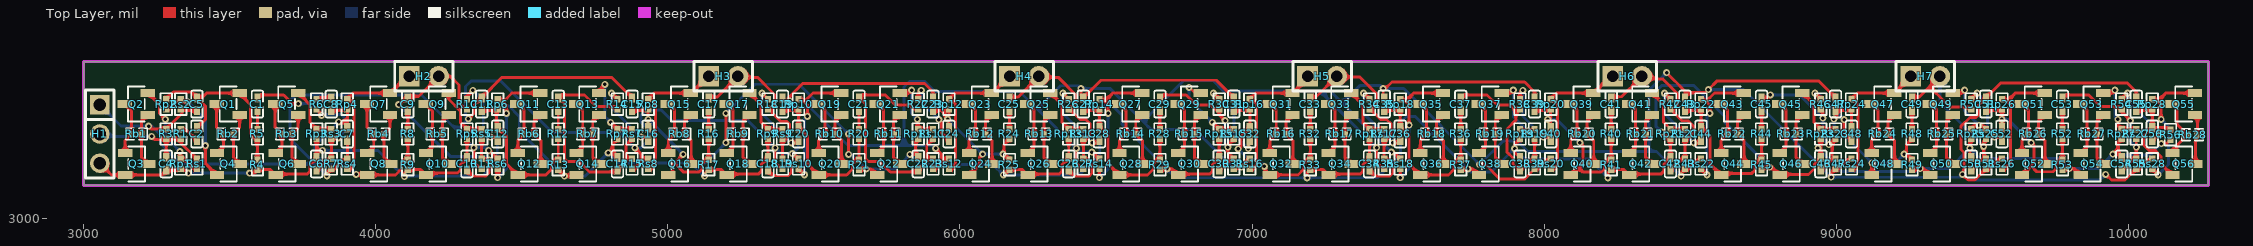
[diagram p0: Top Layer view]
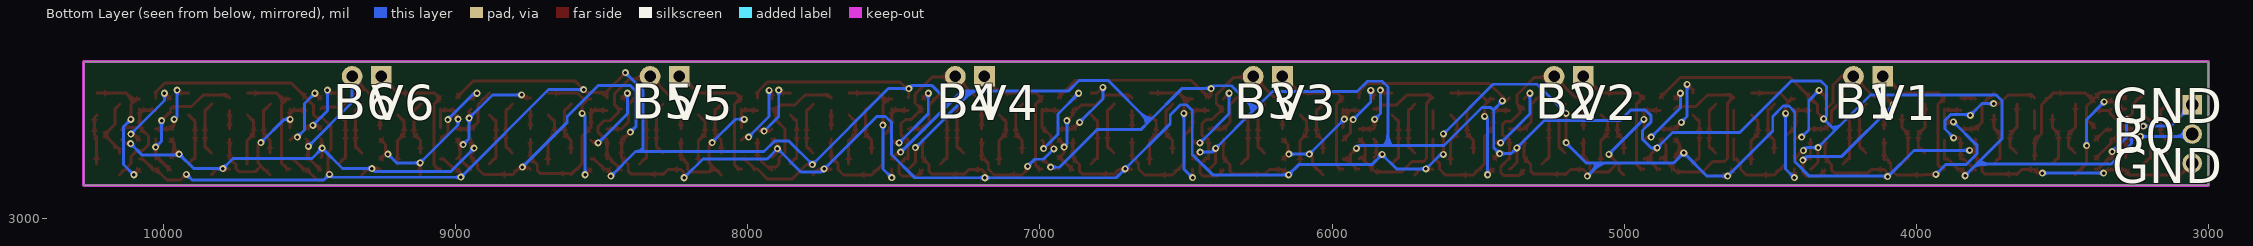
[diagram p1: Bottom Layer view, seen from below]
# Altium PCB MISC51432.pcbdoc (part 1 of 2)
Units mil, origin at the board's own origin, x right, y up, seen from the top; angles counter-clockwise.
Board outline 7274.02 x 423.7 mil, 2 copper layers (Top Layer, Bottom Layer), stack 62.206 mil thick; 257 components, 141 nets, 571 pads, 133 vias.

## Layer stack, top to bottom
Top Solder Mask Layer: solder mask 0.394, Dk 3.3
Top Layer: signal copper 1.379
Dielectric1: surface 59.449, FR4, Dk 4.5
Bottom Layer: signal copper 1.378
Bottom Solder Mask Layer: solder mask 0.394, Dk 3.3

## Board outline
3000,3536.14 3000,3112.44 10274.02,3112.44 10274.02,3536.14

## Design rules (kind name [scope] priority, off if disabled: settings)
BoardOutlineClearance copperThickness2oz_1 [All] p2 off: genericclearance=7.99 ignorepadtopadclearanceinfootprint=FALSE except(0: Arc-SplitContinuation Track-SplitContinuation SMDPad-SplitContinuation THPad-SplitContinuation Via-SplitContinuation Fill-SplitContinuation Region-SplitContinuation Poly-SplitContinuation Text-SplitContinuation Hole-SplitContinuation; 5.98: Arc-CutoutEdge Track-CutoutEdge SMDPad-CutoutEdge THPad-CutoutEdge Via-CutoutEdge Text-CutoutEdge; 6.9: Hole-OutlineEdge Hole-CutoutEdge; 10: Poly-OutlineEdge Poly-CutoutEdge; 11.81: Arc-OutlineEdge Track-OutlineEdge SMDPad-OutlineEdge THPad-OutlineEdge Via-OutlineEdge Fill-OutlineEdge Region-OutlineEdge Text-OutlineEdge Fill-CutoutEdge Region-CutoutEdge)
BoardOutlineClearance Plane_innerPlane_1 [All] p4 off: genericclearance=4.02 ignorepadtopadclearanceinfootprint=FALSE except(0: Arc-SplitContinuation Track-SplitContinuation SMDPad-SplitContinuation THPad-SplitContinuation Via-SplitContinuation Fill-SplitContinuation Region-SplitContinuation Poly-SplitContinuation Text-SplitContinuation Hole-SplitContinuation; 5.98: Arc-CutoutEdge Track-CutoutEdge SMDPad-CutoutEdge THPad-CutoutEdge Via-CutoutEdge Text-CutoutEdge; 6.9: Hole-OutlineEdge Hole-CutoutEdge; 10: Poly-OutlineEdge Poly-CutoutEdge; 11.81: Arc-OutlineEdge Track-OutlineEdge SMDPad-OutlineEdge THPad-OutlineEdge Via-OutlineEdge Fill-OutlineEdge Region-OutlineEdge Text-OutlineEdge Fill-CutoutEdge Region-CutoutEdge)
BoardOutlineClearance Copper_copperRegion_1 [All] p6 off: genericclearance=4.02 ignorepadtopadclearanceinfootprint=FALSE except(0: Arc-SplitContinuation Track-SplitContinuation SMDPad-SplitContinuation THPad-SplitContinuation Via-SplitContinuation Fill-SplitContinuation Region-SplitContinuation Poly-SplitContinuation Text-SplitContinuation Hole-SplitContinuation; 5.98: Arc-CutoutEdge Track-CutoutEdge SMDPad-CutoutEdge THPad-CutoutEdge Via-CutoutEdge Text-CutoutEdge; 6.9: Hole-OutlineEdge Hole-CutoutEdge; 10: Poly-OutlineEdge Poly-CutoutEdge; 11.81: Arc-OutlineEdge Track-OutlineEdge SMDPad-OutlineEdge THPad-OutlineEdge Via-OutlineEdge Fill-OutlineEdge Region-OutlineEdge Text-OutlineEdge Fill-CutoutEdge Region-CutoutEdge)
BoardOutlineClearance copperThickness1oz_1 [All] p8: genericclearance=4.02 ignorepadtopadclearanceinfootprint=FALSE except(0: Arc-SplitContinuation Track-SplitContinuation SMDPad-SplitContinuation THPad-SplitContinuation Via-SplitContinuation Fill-SplitContinuation Region-SplitContinuation Poly-SplitContinuation Text-SplitContinuation Hole-SplitContinuation; 5.98: Arc-CutoutEdge Track-CutoutEdge SMDPad-CutoutEdge THPad-CutoutEdge Via-CutoutEdge Text-CutoutEdge; 6.9: Hole-OutlineEdge Hole-CutoutEdge; 10: Poly-OutlineEdge Poly-CutoutEdge; 11.81: Arc-OutlineEdge Track-OutlineEdge SMDPad-OutlineEdge THPad-OutlineEdge Via-OutlineEdge Fill-OutlineEdge Region-OutlineEdge Text-OutlineEdge Fill-CutoutEdge Region-CutoutEdge)
Clearance copperThickness2oz [All] p1 off: gap=7.99 ignorepadtopadclearanceinfootprint=FALSE except(5.98: SMDPad-Track SMDPad-SMDPad THPad-Track SMDPad-THPad THPad-THPad Track-Via SMDPad-Via THPad-Via Via-Via Fill-SMDPad Region-SMDPad Fill-THPad Region-THPad Fill-Via Region-Via Fill-Fill Fill-Region Region-Region Arc-Track Arc-SMDPad Arc-THPad Arc-Via Fill-Arc Region-Arc Arc-Arc Text-Track SMDPad-Text Text-THPad Text-Via Fill-Text Region-Text Arc-Text Text-Text; 6.9: Hole-Track Hole-SMDPad Hole-THPad Hole-Via Fill-Hole Region-Hole Hole-Arc Hole-Text; 10: Poly-Track Poly-SMDPad Poly-THPad Poly-Via Poly-Fill Poly-Region Poly-Poly Poly-Arc Poly-Text Poly-Hole; 11.81: Fill-Track Region-Track)
Clearance Plane_innerPlane [All] p3 off: gap=4.02 ignorepadtopadclearanceinfootprint=FALSE except(5.98: SMDPad-Track SMDPad-SMDPad THPad-Track SMDPad-THPad THPad-THPad Track-Via SMDPad-Via THPad-Via Via-Via Fill-SMDPad Region-SMDPad Fill-THPad Region-THPad Fill-Via Region-Via Fill-Fill Fill-Region Region-Region Arc-Track Arc-SMDPad Arc-THPad Arc-Via Fill-Arc Region-Arc Arc-Arc Text-Track SMDPad-Text Text-THPad Text-Via Fill-Text Region-Text Arc-Text Text-Text; 6.9: Hole-Track Hole-SMDPad Hole-THPad Hole-Via Fill-Hole Region-Hole Hole-Arc Hole-Text; 10: Poly-Track Poly-SMDPad Poly-THPad Poly-Via Poly-Fill Poly-Region Poly-Poly Poly-Arc Poly-Text Poly-Hole; 11.81: Fill-Track Region-Track)
Clearance Copper_copperRegion [All] p5 off: gap=4.02 ignorepadtopadclearanceinfootprint=FALSE except(5.98: SMDPad-Track SMDPad-SMDPad THPad-Track SMDPad-THPad THPad-THPad Track-Via SMDPad-Via THPad-Via Via-Via Fill-SMDPad Region-SMDPad Fill-THPad Region-THPad Fill-Via Region-Via Fill-Fill Fill-Region Region-Region Arc-Track Arc-SMDPad Arc-THPad Arc-Via Fill-Arc Region-Arc Arc-Arc Text-Track SMDPad-Text Text-THPad Text-Via Fill-Text Region-Text Arc-Text Text-Text; 6.9: Hole-Track Hole-SMDPad Hole-THPad Hole-Via Fill-Hole Region-Hole Hole-Arc Hole-Text; 10: Poly-Track Poly-SMDPad Poly-THPad Poly-Via Poly-Fill Poly-Region Poly-Poly Poly-Arc Poly-Text Poly-Hole; 11.81: Fill-Track Region-Track)
Clearance copperThickness1oz [All] p7: gap=4.02 ignorepadtopadclearanceinfootprint=FALSE except(5.98: SMDPad-Track SMDPad-SMDPad THPad-Track SMDPad-THPad THPad-THPad Track-Via SMDPad-Via THPad-Via Via-Via Fill-SMDPad Region-SMDPad Fill-THPad Region-THPad Fill-Via Region-Via Fill-Fill Fill-Region Region-Region Arc-Track Arc-SMDPad Arc-THPad Arc-Via Fill-Arc Region-Arc Arc-Arc Text-Track SMDPad-Text Text-THPad Text-Via Fill-Text Region-Text Arc-Text Text-Text; 6.9: Hole-Track Hole-SMDPad Hole-THPad Hole-Via Fill-Hole Region-Hole Hole-Arc Hole-Text; 10: Poly-Track Poly-SMDPad Poly-THPad Poly-Via Poly-Fill Poly-Region Poly-Poly Poly-Arc Poly-Text Poly-Hole; 11.81: Fill-Track Region-Track)
DiffPairsRouting differentialPair [All] p1: maxlimit=6 minlimit=6 mostfreqgap=6 toplayer_minwidth=5 toplayer_prefwidth=10 toplayer_maxwidth=100 toplayer_mingap=6 toplayer_prefgap=6 toplayer_maxgap=6 bottomlayer_minwidth=5 bottomlayer_prefwidth=10 bottomlayer_maxwidth=100 bottomlayer_mingap=6 bottomlayer_prefgap=6 bottomlayer_maxgap=6 maxuncoupledlength=10
HoleToHoleClearance otherClearance [All] p1: gap=11.81 allowstackedmicrovias=TRUE
Length netLength [All] p1: minlimit=0 maxlimit=0
PasteMaskExpansion pasteMaskExpansion [All] p1: expansion=0
PlaneConnect innerPlane [All] p1: planeconnectstyle=Relief reliefexpansion=20 reliefentries=4 reliefconductorwidth=10 reliefairgap=10
PolygonConnect copperRegion [All] p1: connectstyle=Relief reliefconductorwidth=10 reliefentries=4 polygonreliefangle="90 Angle" airgapwidth=10 via.connectstyle=Relief via.reliefconductorwidth=10 via.reliefentries=4 via.polygonreliefangle="90 Angle" via.airgapwidth=10
RoutingVias viaSize [All] p1: holewidth=12.01 width=24.02 viastyle="Through Hole" minholewidth=11.81 minwidth=19.68 maxholewidth=248.03 maxwidth=393.7
SolderMaskExpansion solderMaskExpansion [IsVia] p1: expansion=-1000 istentingtop=TRUE
SolderMaskExpansion solderMaskExpansion [All] p2: expansion=2 istentingtop=FALSE
Width copperThickness2oz_2 [All] p1 off: maxlimit=100 minlimit=8 preferedwidth=10
Width copperThickness1oz_2 [All] p2: maxlimit=100 minlimit=5 preferedwidth=10

## Components (designator, comment, footprint, x,y, rotation, side; value= is the part's Value field where it differs from the comment)
C1 "0.1uF" C0402 3594.62,3391.14 r270 top
C2 "0.1uF" C0402 3387.5,3288.64 r270 top
C4 "0.1uF" C0402 3282.5,3186.14 r90 top
C5 "0.1uF" C0402 3387.5,3391.14 r270 top
C6 "0.1uF" C0402 3797.5,3186.14 r270 top
C7 "0.1uF" C0402 3902.5,3288.64 r270 top
C8 "0.1uF" C0402 3847.5,3391.14 r90 top
C9 "0.1uF" C0402 4109.62,3391.14 r270 top
C10 "0.1uF" C0402 4312.5,3186.14 r270 top
C11 "0.1uF" C0402 4362.5,3391.14 r90 top
C12 "0.1uF" C0402 4417.5,3288.64 r270 top
C13 "0.1uF" C0402 4624.62,3391.14 r270 top
C14 "0.1uF" C0402 4827.5,3186.14 r270 top
C15 "0.1uF" C0402 4877.5,3391.14 r90 top
C16 "0.1uF" C0402 4932.5,3288.64 r270 top
C17 "0.1uF" C0402 5139.62,3391.14 r270 top
C18 "0.1uF" C0402 5342.5,3186.14 r270 top
C19 "0.1uF" C0402 5392.5,3391.14 r90 top
C20 "0.1uF" C0402 5447.5,3288.64 r270 top
C21 "0.1uF" C0402 5654.62,3391.14 r270 top
C22 "0.1uF" C0402 5857.5,3186.14 r270 top
C23 "0.1uF" C0402 5907.5,3391.14 r90 top
C24 "0.1uF" C0402 5962.5,3288.64 r270 top
C25 "0.1uF" C0402 6169.62,3391.14 r270 top
C26 "0.1uF" C0402 6372.5,3186.14 r270 top
C27 "0.1uF" C0402 6422.5,3391.14 r90 top
C28 "0.1uF" C0402 6477.5,3288.64 r270 top
C29 "0.1uF" C0402 6684.62,3391.14 r270 top
C30 "0.1uF" C0402 6887.5,3186.14 r270 top
C31 "0.1uF" C0402 6937.5,3391.14 r90 top
C32 "0.1uF" C0402 6992.5,3288.64 r270 top
C33 "0.1uF" C0402 7199.62,3391.14 r270 top
C34 "0.1uF" C0402 7402.5,3186.14 r270 top
C35 "0.1uF" C0402 7452.5,3391.14 r90 top
C36 "0.1uF" C0402 7507.5,3288.64 r270 top
C37 "0.1uF" C0402 7714.62,3391.14 r270 top
C38 "0.1uF" C0402 7917.5,3186.14 r270 top
C39 "0.1uF" C0402 7967.5,3391.14 r90 top
C40 "0.1uF" C0402 8022.5,3288.64 r270 top
C41 "0.1uF" C0402 8229.62,3391.14 r270 top
C42 "0.1uF" C0402 8432.5,3186.14 r270 top
C43 "0.1uF" C0402 8482.5,3391.14 r90 top
C44 "0.1uF" C0402 8537.5,3288.64 r270 top
C45 "0.1uF" C0402 8744.62,3391.14 r270 top
C46 "0.1uF" C0402 8947.5,3186.14 r270 top
C47 "0.1uF" C0402 8997.5,3391.14 r90 top
C48 "0.1uF" C0402 9052.5,3288.64 r270 top
C49 "0.1uF" C0402 9259.62,3391.14 r270 top
C50 "0.1uF" C0402 9462.5,3186.14 r270 top
C51 "0.1uF" C0402 9512.5,3391.14 r90 top
C52 "0.1uF" C0402 9567.5,3288.64 r270 top
C53 "0.1uF" C0402 9774.62,3391.14 r270 top
C54 "0.1uF" C0402 9977.5,3186.14 r270 top
C55 "0.1uF" C0402 10027.5,3391.14 r90 top
C56 "0.1uF" C0402 10082.5,3288.64 r270 top
H1 "" HDR-TH_3P-P2.54-V-M 3055,3288.64 r270 top
H2 "" HDR-TH_2P-P2.54-V-M-1 4165,3486.14 r0 top
H3 "" HDR-TH_2P-P2.54-V-M-1 5190,3486.14 r0 top
H4 "" HDR-TH_2P-P2.54-V-M-1 6220,3486.14 r0 top
H5 "" HDR-TH_2P-P2.54-V-M-1 7240,3486.14 r0 top
H6 "" HDR-TH_2P-P2.54-V-M-1 8285,3486.14 r0 top
H7 "" HDR-TH_2P-P2.54-V-M-1 9305,3486.14 r0 top
Q1 "MMBT3906" SOT-23-3_L2.9-W1.3-P1.90-LS2.4-BR 3494.31,3391.14 r0 top
Q2 "MMBT3904" SOT-23-3_L2.9-W1.3-P1.90-LS2.4-BR 3180,3391.14 r0 top
Q3 "MMBT3906" SOT-23-3_L2.9-W1.3-P1.90-LS2.4-BR 3181.38,3186.14 r180 top
Q4 "MMBT3904" SOT-23-3_L2.9-W1.3-P1.90-LS2.4-BR 3495.69,3186.14 r180 top
Q5 "MMBT3904" SOT-23-3_L2.9-W1.3-P1.90-LS2.4-BR 3695,3391.14 r0 top
Q6 "MMBT3906" SOT-23-3_L2.9-W1.3-P1.90-LS2.4-BR 3696.38,3186.14 r180 top
Q7 "MMBT3904" SOT-23-3_L2.9-W1.3-P1.90-LS2.4-BR 4009.31,3391.14 r0 top
Q8 "MMBT3906" SOT-23-3_L2.9-W1.3-P1.90-LS2.4-BR 4010.69,3186.14 r180 top
Q9 "MMBT3904" SOT-23-3_L2.9-W1.3-P1.90-LS2.4-BR 4210,3391.14 r0 top
Q10 "MMBT3906" SOT-23-3_L2.9-W1.3-P1.90-LS2.4-BR 4211.38,3186.14 r180 top
Q11 "MMBT3904" SOT-23-3_L2.9-W1.3-P1.90-LS2.4-BR 4524.31,3391.14 r0 top
Q12 "MMBT3906" SOT-23-3_L2.9-W1.3-P1.90-LS2.4-BR 4525.69,3186.14 r180 top
Q13 "MMBT3904" SOT-23-3_L2.9-W1.3-P1.90-LS2.4-BR 4725,3391.14 r0 top
Q14 "MMBT3906" SOT-23-3_L2.9-W1.3-P1.90-LS2.4-BR 4726.38,3186.14 r180 top
Q15 "MMBT3904" SOT-23-3_L2.9-W1.3-P1.90-LS2.4-BR 5039.31,3391.14 r0 top
Q16 "MMBT3906" SOT-23-3_L2.9-W1.3-P1.90-LS2.4-BR 5040.69,3186.14 r180 top
Q17 "MMBT3904" SOT-23-3_L2.9-W1.3-P1.90-LS2.4-BR 5240,3391.14 r0 top
Q18 "MMBT3906" SOT-23-3_L2.9-W1.3-P1.90-LS2.4-BR 5241.38,3186.14 r180 top
Q19 "MMBT3904" SOT-23-3_L2.9-W1.3-P1.90-LS2.4-BR 5554.31,3391.14 r0 top
Q20 "MMBT3906" SOT-23-3_L2.9-W1.3-P1.90-LS2.4-BR 5555.69,3186.14 r180 top
Q21 "MMBT3904" SOT-23-3_L2.9-W1.3-P1.90-LS2.4-BR 5755,3391.14 r0 top
Q22 "MMBT3906" SOT-23-3_L2.9-W1.3-P1.90-LS2.4-BR 5756.38,3186.14 r180 top
Q23 "MMBT3904" SOT-23-3_L2.9-W1.3-P1.90-LS2.4-BR 6069.31,3391.14 r0 top
Q24 "MMBT3906" SOT-23-3_L2.9-W1.3-P1.90-LS2.4-BR 6070.69,3186.14 r180 top
Q25 "MMBT3904" SOT-23-3_L2.9-W1.3-P1.90-LS2.4-BR 6270,3391.14 r0 top
Q26 "MMBT3906" SOT-23-3_L2.9-W1.3-P1.90-LS2.4-BR 6271.38,3186.14 r180 top
Q27 "MMBT3904" SOT-23-3_L2.9-W1.3-P1.90-LS2.4-BR 6584.31,3391.14 r0 top
Q28 "MMBT3906" SOT-23-3_L2.9-W1.3-P1.90-LS2.4-BR 6585.69,3186.14 r180 top
Q29 "MMBT3904" SOT-23-3_L2.9-W1.3-P1.90-LS2.4-BR 6785,3391.14 r0 top
Q30 "MMBT3906" SOT-23-3_L2.9-W1.3-P1.90-LS2.4-BR 6786.38,3186.14 r180 top
Q31 "MMBT3904" SOT-23-3_L2.9-W1.3-P1.90-LS2.4-BR 7099.31,3391.14 r0 top
Q32 "MMBT3906" SOT-23-3_L2.9-W1.3-P1.90-LS2.4-BR 7100.69,3186.14 r180 top
Q33 "MMBT3904" SOT-23-3_L2.9-W1.3-P1.90-LS2.4-BR 7300,3391.14 r0 top
Q34 "MMBT3906" SOT-23-3_L2.9-W1.3-P1.90-LS2.4-BR 7301.38,3186.14 r180 top
Q35 "MMBT3904" SOT-23-3_L2.9-W1.3-P1.90-LS2.4-BR 7614.31,3391.14 r0 top
Q36 "MMBT3906" SOT-23-3_L2.9-W1.3-P1.90-LS2.4-BR 7615.69,3186.14 r180 top
Q37 "MMBT3904" SOT-23-3_L2.9-W1.3-P1.90-LS2.4-BR 7815,3391.14 r0 top
Q38 "MMBT3906" SOT-23-3_L2.9-W1.3-P1.90-LS2.4-BR 7816.38,3186.14 r180 top
Q39 "MMBT3904" SOT-23-3_L2.9-W1.3-P1.90-LS2.4-BR 8129.31,3391.14 r0 top
Q40 "MMBT3906" SOT-23-3_L2.9-W1.3-P1.90-LS2.4-BR 8130.69,3186.14 r180 top
Q41 "MMBT3904" SOT-23-3_L2.9-W1.3-P1.90-LS2.4-BR 8330,3391.14 r0 top
Q42 "MMBT3906" SOT-23-3_L2.9-W1.3-P1.90-LS2.4-BR 8331.38,3186.14 r180 top
Q43 "MMBT3904" SOT-23-3_L2.9-W1.3-P1.90-LS2.4-BR 8644.31,3391.14 r0 top
Q44 "MMBT3906" SOT-23-3_L2.9-W1.3-P1.90-LS2.4-BR 8645.69,3186.14 r180 top
Q45 "MMBT3904" SOT-23-3_L2.9-W1.3-P1.90-LS2.4-BR 8845,3391.14 r0 top
Q46 "MMBT3906" SOT-23-3_L2.9-W1.3-P1.90-LS2.4-BR 8846.38,3186.14 r180 top
Q47 "MMBT3904" SOT-23-3_L2.9-W1.3-P1.90-LS2.4-BR 9159.31,3391.14 r0 top
Q48 "MMBT3906" SOT-23-3_L2.9-W1.3-P1.90-LS2.4-BR 9160.69,3186.14 r180 top
Q49 "MMBT3904" SOT-23-3_L2.9-W1.3-P1.90-LS2.4-BR 9360,3391.14 r0 top
Q50 "MMBT3906" SOT-23-3_L2.9-W1.3-P1.90-LS2.4-BR 9361.38,3186.14 r180 top
Q51 "MMBT3904" SOT-23-3_L2.9-W1.3-P1.90-LS2.4-BR 9674.31,3391.14 r0 top
Q52 "MMBT3906" SOT-23-3_L2.9-W1.3-P1.90-LS2.4-BR 9675.69,3186.14 r180 top
Q53 "MMBT3904" SOT-23-3_L2.9-W1.3-P1.90-LS2.4-BR 9875,3391.14 r0 top
Q54 "MMBT3906" SOT-23-3_L2.9-W1.3-P1.90-LS2.4-BR 9876.38,3186.14 r180 top
Q55 "MMBT3904" SOT-23-3_L2.9-W1.3-P1.90-LS2.4-BR 10189.31,3391.14 r0 top
Q56 "MMBT3906" SOT-23-3_L2.9-W1.3-P1.90-LS2.4-BR 10190.69,3186.14 r180 top
R1 "1" R0402 3332.5,3288.64 r270 top
R3 "2.2K" R0402 3282.5,3288.64 r90 top
R4 "2.2K" R0402 3594.62,3184.1 r90 top
R5 "1" R0402 3594.62,3288.64 r270 top
R6 "1" R0402 3797.5,3391.14 r270 top
R7 "2.2K" R0402 3847.5,3186.14 r270 top
R8 "1" R0402 4109.62,3288.64 r270 top
R9 "2.2K" R0402 4109.62,3184.1 r90 top
R10 "1" R0402 4312.5,3391.14 r270 top
R11 "2.2K" R0402 4362.5,3186.14 r270 top
R12 "1" R0402 4624.62,3288.64 r270 top
R13 "2.2K" R0402 4624.62,3184.1 r90 top
R14 "1" R0402 4827.5,3391.14 r270 top
R15 "2.2K" R0402 4877.5,3186.14 r270 top
R16 "1" R0402 5139.62,3288.64 r270 top
R17 "2.2K" R0402 5139.62,3184.1 r90 top
R18 "1" R0402 5342.5,3391.14 r270 top
R19 "2.2K" R0402 5392.5,3186.14 r270 top
R20 "1" R0402 5654.62,3288.64 r270 top
R21 "2.2K" R0402 5654.62,3184.1 r90 top
R22 "1" R0402 5857.5,3391.14 r270 top
R23 "2.2K" R0402 5907.5,3186.14 r270 top
R24 "1" R0402 6169.62,3288.64 r270 top
R25 "2.2K" R0402 6169.62,3184.1 r90 top
R26 "1" R0402 6372.5,3391.14 r270 top
R27 "2.2K" R0402 6422.5,3186.14 r270 top
R28 "1" R0402 6684.62,3288.64 r270 top
R29 "2.2K" R0402 6684.62,3184.1 r90 top
R30 "1" R0402 6887.5,3391.14 r270 top
R31 "2.2K" R0402 6937.5,3186.14 r270 top
R32 "1" R0402 7199.62,3288.64 r270 top
R33 "2.2K" R0402 7199.62,3184.1 r90 top
R34 "1" R0402 7402.5,3391.14 r270 top
R35 "2.2K" R0402 7452.5,3186.14 r270 top
R36 "1" R0402 7714.62,3288.64 r270 top
R37 "2.2K" R0402 7714.62,3184.1 r90 top
R38 "1" R0402 7917.5,3391.14 r270 top
R39 "2.2K" R0402 7967.5,3186.14 r270 top
R40 "1" R0402 8229.62,3288.64 r270 top
R41 "2.2K" R0402 8229.62,3184.1 r90 top
R42 "1" R0402 8432.5,3391.14 r270 top
R43 "2.2K" R0402 8482.5,3186.14 r270 top
R44 "1" R0402 8744.62,3288.64 r270 top
R45 "2.2K" R0402 8744.62,3184.1 r90 top
R46 "1" R0402 8947.5,3391.14 r270 top
R47 "2.2K" R0402 8997.5,3186.14 r270 top
R48 "1" R0402 9259.62,3288.64 r270 top
R49 "2.2K" R0402 9259.62,3184.1 r90 top
R50 "1" R0402 9462.5,3391.14 r270 top
R51 "2.2K" R0402 9512.5,3186.14 r270 top
R52 "1" R0402 9774.62,3288.64 r270 top
R53 "2.2K" R0402 9774.62,3184.1 r90 top
R54 "1" R0402 9977.5,3391.14 r270 top
R55 "2.2K" R0402 10027.5,3186.14 r270 top
R56 "2.2K" R0402 10145,3286.14 r90 top
Rb1 "1K" R0402 3180.69,3288.64 r180 top
Rb2 "1K" R0402 3495,3288.64 r0 top
Rb3 "1K" R0402 3695.69,3288.64 r180 top
Rb4 "1K" R0402 4010,3288.64 r180 top
Rb5 "1K" R0402 4210.69,3288.64 r180 top
Rb6 "1K" R0402 4525,3288.64 r180 top
Rb7 "1K" R0402 4725.69,3288.64 r180 top
Rb8 "1K" R0402 5040,3288.64 r180 top
Rb9 "1K" R0402 5240.69,3288.64 r180 top
Rb10 "1K" R0402 5555,3288.64 r180 top
Rb11 "1K" R0402 5755.69,3288.64 r180 top
Rb12 "1K" R0402 6070,3288.64 r180 top
Rb13 "1K" R0402 6270.69,3288.64 r180 top
Rb14 "1K" R0402 6585,3288.64 r180 top
Rb15 "1K" R0402 6785.69,3288.64 r180 top
Rb16 "1K" R0402 7100,3288.64 r180 top
Rb17 "1K" R0402 7300.69,3288.64 r180 top
Rb18 "1K" R0402 7615,3288.64 r180 top
Rb19 "1K" R0402 7815.69,3288.64 r180 top
Rb20 "1K" R0402 8130,3288.64 r180 top
Rb21 "1K" R0402 8330.69,3288.64 r180 top
Rb22 "1K" R0402 8645,3288.64 r180 top
Rb23 "1K" R0402 8845.69,3288.64 r180 top
Rb24 "1K" R0402 9160,3288.64 r180 top
Rb25 "1K" R0402 9360.69,3288.64 r180 top
Rb26 "1K" R0402 9675,3288.64 r180 top
Rb27 "1K" R0402 9875.69,3288.64 r180 top
Rb28 "1K" R0402 10220,3286.14 r180 top
Rp1 "200K" R0402 3332.5,3186.14 r90 top
Rp2 "200K" R0402 3282.5,3391.14 r270 top
Rp3 "200K" R0402 3797.5,3288.64 r90 top
Rp4 "200K" R0402 3902.5,3391.14 r90 top
Rp5 "200K" R0402 4312.5,3288.64 r90 top
Rp6 "200K" R0402 4417.5,3391.14 r90 top
Rp7 "200K" R0402 4827.5,3288.64 r90 top
Rp8 "200K" R0402 4932.5,3391.14 r90 top
Rp9 "200K" R0402 5342.5,3288.64 r90 top
Rp10 "200K" R0402 5447.5,3391.14 r90 top
Rp11 "200K" R0402 5857.5,3288.64 r90 top
Rp12 "200K" R0402 5962.5,3391.14 r90 top
Rp13 "200K" R0402 6372.5,3288.64 r90 top
Rp14 "200K" R0402 6477.5,3391.14 r90 top
Rp15 "200K" R0402 6887.5,3288.64 r90 top
Rp16 "200K" R0402 6992.5,3391.14 r90 top
Rp17 "200K" R0402 7402.5,3288.64 r90 top
Rp18 "200K" R0402 7507.5,3391.14 r90 top
Rp19 "200K" R0402 7917.5,3288.64 r90 top
Rp20 "200K" R0402 8022.5,3391.14 r90 top
Rp21 "200K" R0402 8432.5,3288.64 r90 top
Rp22 "200K" R0402 8537.5,3391.14 r90 top
Rp23 "200K" R0402 8947.5,3288.64 r90 top
Rp24 "200K" R0402 9052.5,3391.14 r90 top
Rp25 "200K" R0402 9462.5,3288.64 r90 top
Rp26 "200K" R0402 9567.5,3391.14 r90 top
Rp27 "200K" R0402 9977.5,3288.64 r90 top
Rp28 "200K" R0402 10082.5,3391.14 r90 top
Rs1 "200" R0402 3387.5,3186.14 r90 top
Rs2 "200" R0402 3332.5,3391.14 r270 top
Rs3 "200" R0402 3847.5,3288.64 r270 top
Rs4 "200" R0402 3902.5,3186.14 r90 top
Rs5 "200" R0402 4362.5,3288.64 r270 top
Rs6 "200" R0402 4417.5,3186.14 r90 top
Rs7 "200" R0402 4877.5,3288.64 r270 top
Rs8 "200" R0402 4932.5,3186.14 r90 top
Rs9 "200" R0402 5392.5,3288.64 r270 top
Rs10 "200" R0402 5447.5,3186.14 r90 top
Rs11 "200" R0402 5907.5,3288.64 r270 top
Rs12 "200" R0402 5962.5,3186.14 r90 top
Rs13 "200" R0402 6422.5,3288.64 r270 top
Rs14 "200" R0402 6477.5,3186.14 r90 top
Rs15 "200" R0402 6937.5,3288.64 r270 top
Rs16 "200" R0402 6992.5,3186.14 r90 top
Rs17 "200" R0402 7452.5,3288.64 r270 top
Rs18 "200" R0402 7507.5,3186.14 r90 top
Rs19 "200" R0402 7967.5,3288.64 r270 top
Rs20 "200" R0402 8022.5,3186.14 r90 top
Rs21 "200" R0402 8482.5,3288.64 r270 top
Rs22 "200" R0402 8537.5,3186.14 r90 top
Rs23 "200" R0402 8997.5,3288.64 r270 top
Rs24 "200" R0402 9052.5,3186.14 r90 top
Rs25 "200" R0402 9512.5,3288.64 r270 top
Rs26 "200" R0402 9567.5,3186.14 r90 top
Rs27 "200" R0402 10027.5,3288.64 r270 top
Rs28 "200" R0402 10082.5,3186.14 r90 top

## Footprints (in the part's own frame and the unit in brackets; to place one, negate y for a bottom-side part, rotate by r counter-clockwise, add the part's x,y. Pads: shape width x height; smd on the part's side, far side on the other; paste and mask are expansions set on the pad)
C0402 [mm]
  rect 0.79x0.54 smd paste-100 mask+0.051: 1(-0.545,0) 2(0.545,0)
  silkscreen extent -1.17,-0.5 1.17,0.5
HDR-TH_2P-P2.54-V-M-1 [mm]
  rect 1.8x1.8 hole 1: 1(-1.27,0)
  round 1.8 hole 1: 2(1.27,0)
  silkscreen extent -2.54,-1.27 2.54,1.27
HDR-TH_3P-P2.54-V-M [mm]
  rect 1.7x1.7 hole 1.1: 1(-2.54,0)
  round 1.7 hole 1.1: 2(0,0) 3(2.54,0)
  silkscreen extent -3.81,-1.25 3.81,1.25
R0402 [mm]
  rect 0.566x0.54 smd paste-100 mask+0.051: 1(-0.433,0) 2(0.433,0)
  silkscreen extent -0.94,-0.5 0.94,0.5
SOT-23-3_L2.9-W1.3-P1.90-LS2.4-BR [mm]
  rect 1.25x0.7 smd: 1(1,-0.95) 2(1,0.95) 3(-1,0)
  silkscreen extent -0.73,-1.53 0.73,1.53

## Via types
v1: diameter 24.02, hole 12, Top Layer to Bottom Layer, 133 vias

## Nets (pads, with @x,y where several pads share a name; then routed paths per layer and width w, separated by ;. In a path a pad name is that pad's centre, name@x,y a point inside that pad or via, vN(x,y) a via of type N, cw(c..) or ccw(c..) an arc to the next point about the centre after c; other vN are vias at no path point)
$1N718: Q2.3 Q3.1 Rb1.2 | length 186.3
  Top Layer w10: Q2.3@3140.63,3391.14 3163.22,3368.55 Rb1.2@3163.22,3288.21 ; Q3.1@3142.01,3223.54 3142.01,3267 Rb1.2@3163.22,3288.21 ; Rb1.2@3163.65,3288.64 Rb1.2@3163.22,3288.21
$1N762: Q2.1 Q3.3 Rb1.1 | length 186.1
  Top Layer w10: Q2.1@3219.37,3353.74 3197.73,3332.1 Rb1.1@3197.73,3288.64 3197.73,3209.16 Q3.3@3220.75,3186.14
$1N871: C4.1 C6.1 C10.1 C14.1 C18.1 C22.1 C26.1 C30.1 C34.1 C38.1 C42.1 C46.1 C50.1 C54.1 H1.3 Q3.2 Q6.2 Q10.2 Q14.2 Q18.2 Q22.2 Q26.2 Q30.2 Q34.2 Q38.2 Q42.2 Q46.2 Q50.2 Q54.2 R4.1 R9.1 R13.1 R17.1 R21.1 R25.1 R29.1 R33.1 R37.1 R41.1 R45.1 R49.1 R53.1 R56.1 Rp1.1 Rp3.1 Rp5.1 Rp7.1 Rp9.1 Rp11.1 Rp13.1 Rp15.1 Rp17.1 Rp19.1 Rp21.1 Rp23.1 Rp25.1 Rp27.1 | length 12003.2
  Top Layer w10: H1.3@3055,3188.64 3094.9,3148.74 Q3.2@3142.01,3148.74 3269.06,3148.74 C4.1@3285,3164.68 ; C4.1@3282.5,3164.68 C4.1@3285,3164.68 ; Rp1.1@3332.5,3169.1 Rp1.1@3328.08,3164.68 ; v1(3358.08,3154.68) 3348.08,3164.68 Rp1.1@3328.08,3164.68 ; v1(3568.08,3154.68) 3582.24,3154.68 R4.1@3594.62,3167.06 3638.69,3167.06 Q6.2@3654.6,3151.15 ; Q6.2@3657.01,3148.74 Q6.2@3654.6,3151.15 ; Rp3.1@3797.5,3271.6 3797.5,3232.6 ; v1(3817.5,3232.6) 3797.5,3232.6 ; v1(4097.5,3142.6) 4097.5,3154.94 R9.1@4109.62,3167.06 4153.69,3167.06 Q10.2@4166.06,3154.69 ; Q10.2@4172.01,3148.74 Q10.2@4166.06,3154.69 ; Rp5.1@4312.5,3271.6 C10.1@4312.5,3207.6 4289.59,3184.69 4289.59,3164.69 4279.59,3154.69 Q10.2@4166.06,3154.69 ; R13.1@4624.62,3167.06 v1@4645.89,3145.79 ; v1(4645.89,3144.21) v1@4645.89,3145.79 ; Q14.2@4687.01,3148.74 4684.06,3145.79 v1@4645.89,3145.79 ; v1(4795.89,3224.21) 4810.89,3224.21 ; C14.1@4827.5,3207.6 4810.89,3224.21 ; Rp7.1@4827.5,3271.6 4810.89,3254.99 4810.89,3224.21 ; v1(5125.89,3144.21) 5125.89,3153.33 R17.1@5139.62,3167.06 5183.69,3167.06 Q18.2@5199.6,3151.15 ; v1(5198.74,3258.86) v1(5198.74,3358.86) ; Q18.2@5202.01,3148.74 Q18.2@5199.6,3151.15 ; Rp9.1@5342.5,3271.6 C18.1@5342.5,3207.6 5319.6,3184.7 5319.6,3161.15 5309.6,3151.15 Q18.2@5199.6,3151.15 ; v1(5618.74,3218.86) v1(5618.74,3288.86) ; R21.1@5654.62,3167.06 5656.41,3168.86 v1(5678.74,3168.86) 5696.89,3168.86 Q22.2@5717.01,3148.74 ; v1(5828.74,3218.86) 5846.24,3218.86 C22.1@5848.01,3217.09 ; C22.1@5857.5,3207.6 C22.1@5848.01,3217.09 ; Rp11.1@5857.5,3271.6 5848.01,3262.11 C22.1@5848.01,3217.09 ; v1(6148.74,3148.86) 6151.41,3148.86 R25.1@6169.62,3167.06 6213.69,3167.06 Q26.2@6229.6,3151.15 ; Q26.2@6232.01,3148.74 Q26.2@6229.6,3151.15 ; Rp13.1@6372.5,3271.6 C26.1@6372.5,3207.6 6349.6,3184.7 6349.6,3161.15 6339.6,3151.15 Q26.2@6229.6,3151.15 ; R29.1@6684.62,3167.06 6686.41,3168.86 v1(6708.74,3168.86) 6726.89,3168.86 Q30.2@6744.57,3151.18 ; Q30.2@6747.01,3148.74 Q30.2@6744.57,3151.18 ; Rp15.1@6887.5,3271.6 C30.1@6887.5,3207.6 6864.57,3184.67 6864.57,3161.18 6854.57,3151.18 Q30.2@6744.57,3151.18 ; v1(7188.74,3138.86) 7188.74,3156.19 R33.1@7199.62,3167.06 7243.69,3167.06 Q34.2@7259.6,3151.15 ; Q34.2@7262.01,3148.74 Q34.2@7259.6,3151.15 ; Rp17.1@7402.5,3271.6 C34.1@7402.5,3207.6 7379.6,3184.7 7379.6,3161.15 7369.6,3151.15 Q34.2@7259.6,3151.15 ; R37.1@7714.62,3167.06 7716.41,3168.86 v1(7738.74,3168.86) 7756.89,3168.86 Q38.2@7777.01,3148.74 ; C38.1@7917.5,3207.6 7898.74,3226.36 v1(7898.74,3238.86) 7898.74,3252.84 Rp19.1@7917.5,3271.6 ; v1(8218.74,3138.86) 8218.74,3156.19 R41.1@8229.62,3167.06 8273.69,3167.06 Q42.2@8289.6,3151.15 ; Q42.2@8292.01,3148.74 Q42.2@8289.6,3151.15 ; v1(8402.5,3295.1) Rp21.1@8432.5,3265.1 ; Rp21.1@8432.5,3271.6 Rp21.1@8432.5,3265.1 ; R45.1@8744.62,3167.06 8752.66,3175.1 v1(8772.5,3175.1) 8780.65,3175.1 Q46.2@8805.4,3150.35 ; Q46.2@8807.01,3148.74 Q46.2@8805.4,3150.35 ; v1(8937.5,3240.1) v1@8947.5,3240.1 ; Rp23.1@8947.5,3271.6 v1@8947.5,3240.1 ; R49.1@9259.62,3167.06 9262.66,3170.1 v1(9287.5,3170.1) 9300.65,3170.1 Q50.2@9322.01,3148.74 ; C50.1@9462.5,3207.6 9457.5,3212.6 v1(9457.5,3240.1) 9457.5,3266.6 Rp25.1@9462.5,3271.6 ; R53.1@9774.62,3167.06 9777.66,3170.1 v1(9797.5,3170.1) 9815.65,3170.1 Q54.2@9837.01,3148.74 ; v1(9947.5,3220.1) 9965,3220.1 ; C54.1@9977.5,3207.6 9965,3220.1 ; Rp27.1@9977.5,3271.6 9965,3259.1 9965,3220.1 ; v1(10113.46,3256.06) 10131.96,3256.06 R56.1@10145,3269.1 ; C4.1@3285,3164.68 Rp1.1@3328.08,3164.68 ; Q6.2@3654.6,3151.15 3764.6,3151.15 3774.6,3161.15 3774.6,3184.7 C6.1@3797.5,3207.6 3797.5,3232.6 ; Q42.2@8289.6,3151.15 8399.6,3151.15 8409.6,3161.15 8409.6,3184.7 C42.1@8432.5,3207.6 Rp21.1@8432.5,3265.1 ; Q46.2@8805.4,3150.35 8905.4,3150.35 8925.4,3170.35 8925.4,3185.5 C46.1@8947.5,3207.6 v1@8947.5,3240.1
  Bottom Layer w10: v1(3358.08,3154.68) v1(3568.08,3154.68) ; v1(3817.5,3232.6) 4007.5,3232.6 v1@4095.89,3144.21 ; v1(4097.5,3142.6) v1@4095.89,3144.21 ; v1(5125.89,3144.21) 5081.24,3188.86 ; v1(5198.74,3258.86) 5128.74,3188.86 5081.24,3188.86 ; v1(5198.74,3358.86) 5298.74,3458.86 5448.74,3458.86 v1(5618.74,3288.86) ; v1(5618.74,3218.86) 5628.74,3218.86 v1(5678.74,3168.86) 5778.74,3168.86 v1(5828.74,3218.86) 5864.1,3183.5 6114.1,3183.5 v1(6148.74,3148.86) 6408.74,3148.86 6478.74,3218.86 6478.74,3368.86 6498.74,3388.86 6518.74,3388.86 6554.1,3353.5 6554.1,3323.5 v1(6708.74,3168.86) 6738.74,3138.86 v1(7188.74,3138.86) 7428.74,3138.86 7508.74,3218.86 7508.74,3328.86 7528.74,3348.86 7558.74,3348.86 v1(7738.74,3168.86) 7748.74,3158.86 7818.74,3158.86 v1(7898.74,3238.86) 7934.1,3203.5 8154.1,3203.5 v1(8218.74,3138.86) ; v1(8402.5,3295.1) 8382.5,3315.1 8382.5,3435.1 8402.5,3455.1 8512.5,3455.1 8618.57,3349.03 8618.57,3329.03 v1(8772.5,3175.1) ; v1(8937.5,3240.1) 9017.5,3160.1 9277.5,3160.1 v1(9287.5,3170.1) 9387.5,3170.1 v1(9457.5,3240.1) 9492.85,3204.75 9762.85,3204.75 v1(9797.5,3170.1) 9897.5,3170.1 v1@9943.46,3216.06 ; v1(9947.5,3220.1) v1@9943.46,3216.06 ; v1(10113.46,3256.06) 10073.46,3216.06 v1@9943.46,3216.06 ; v1@4095.89,3144.21 4365.89,3144.21 4415.89,3194.21 4415.89,3364.21 4435.89,3384.21 4455.89,3384.21 4491.24,3348.86 4491.24,3298.86 v1(4645.89,3144.21) 4715.89,3144.21 v1(4795.89,3224.21) 4831.24,3188.86 5081.24,3188.86
$1N1153: Q1.1 Q4.3 Rb2.2 | length 186.3
  Top Layer w10: Rb2.2@3512.04,3288.64 Rb2.2@3512.47,3289.07 ; Q1.1@3533.68,3353.74 3533.68,3310.28 Rb2.2@3512.47,3289.07 ; Q4.3@3535.06,3186.14 3512.47,3208.73 Rb2.2@3512.47,3289.07
$1N1158: Q1.3 Q4.1 Rb2.1 | length 186.1
  Top Layer w10: Q1.3@3454.94,3391.14 3454.94,3311.66 Rb2.1@3477.96,3288.64 3477.96,3245.18 Q4.1@3456.32,3223.54
$1N1224: C2.2 R1.1 | length 70.9
  Top Layer w10: R1.1@3332.5,3305.68 3335.64,3302.54 3352.14,3302.54 C2.2@3387.5,3267.18
$1N1967: C1.1 C6.2 R6.2 R7.1 Rs3.2 | length 613.6
  Top Layer w10: C1.1@3594.62,3412.6 3604.62,3422.6 3684.62,3422.6 3714.62,3392.6 v1(3734.62,3392.6) ; C6.2@3797.5,3164.68 3836.34,3203.52 R7.1@3847.84,3203.52 ; R6.2@3797.5,3374.1 3814.62,3356.98 v1(3814.62,3352.6) ; R7.1@3847.5,3203.18 R7.1@3847.84,3203.52 ; Rs3.2@3847.5,3271.6 Rs3.2@3847.84,3271.94 ; v1(3871.74,3275.48) 3851.38,3275.48 Rs3.2@3847.84,3271.94 ; R7.1@3847.84,3203.52 Rs3.2@3847.84,3271.94
  Bottom Layer w10: v1(3734.62,3392.6) 3774.62,3392.6 v1@3811.74,3355.48 ; v1(3814.62,3352.6) v1@3811.74,3355.48 ; v1(3871.74,3275.48) 3901.74,3305.48 3901.74,3335.48 3881.74,3355.48 v1@3811.74,3355.48
$1N1970: C1.2 R5.1 | length 64
  Top Layer w10: R5.1@3594.62,3305.68 C1.2@3594.62,3369.68
$1N1975: C2.1 C5.1 Q1.2 R4.2 R5.2 Rp2.1 | length 655.9
  Top Layer w10: Rp2.1@3282.5,3408.18 3306.92,3432.6 3367.5,3432.6 C5.1@3387.5,3412.6 C5.1@3396.34,3403.76 ; C2.1@3387.5,3310.1 3417.5,3340.1 3417.5,3382.6 C5.1@3396.34,3403.76 ; Q1.2@3533.68,3428.54 Q1.2@3531.12,3428.54 ; R4.2@3594.62,3201.14 R5.2@3594.62,3271.6 3588.06,3271.6 3571.12,3288.54 3571.12,3388.54 Q1.2@3531.12,3428.54 ; C5.1@3396.34,3403.76 3421.12,3428.54 Q1.2@3531.12,3428.54
$1N3936: C4.2 H1.2 R1.2 R3.1 Rs1.2 | length 440.4
  Top Layer w10: v1(3232.5,3280.1) 3242.5,3270.1 R3.1@3282.5,3270.1 ; C4.2@3282.5,3207.6 R3.1@3282.5,3270.1 ; Rs1.2@3387.5,3203.18 3332.5,3258.18 R1.2@3332.5,3271.6 R3.1@3282.5,3271.6 R3.1@3282.5,3270.1
  Bottom Layer w10: H1.2@3055,3288.64 3063.54,3280.1 v1(3232.5,3280.1)
$1N3942: Q2.2 Rp1.2 Rs1.1 | length 341.3
  Top Layer w10: Q2.2@3219.37,3428.54 3259.37,3388.54 3259.37,3358.54 v1(3279.37,3338.54) ; v1(3329.37,3228.54) 3329.37,3206.31 Rp1.2@3332.5,3203.18 3342.5,3203.18 3376.58,3169.1 Rs1.1@3387.5,3169.1
  Bottom Layer w10: v1(3279.37,3338.54) 3279.37,3278.54 v1(3329.37,3228.54)
$1N4003: Q4.2 Rp2.2 Rs2.1 | length 385
  Top Layer w10: Rp2.2@3282.5,3374.1 3291.68,3374.1 3316.32,3398.74 Rs2.1@3331.32,3398.74 ; Rs2.1@3332.5,3408.18 Rs2.1@3331.32,3398.74 ; v1(3356.32,3398.74) Rs2.1@3331.32,3398.74 ; v1(3416.32,3248.74) 3416.32,3188.74 Q4.2@3456.32,3148.74
  Bottom Layer w10: v1(3356.32,3398.74) 3416.32,3338.74 v1(3416.32,3248.74)
$1N4031: C5.2 C7.2 C11.2 C15.2 C19.2 C23.2 C27.2 C31.2 C35.2 C39.2 C43.2 C47.2 C51.2 C55.2 H1.1 R3.2 R7.2 R11.2 R15.2 R19.2 R23.2 R27.2 R31.2 R35.2 R39.2 R43.2 R47.2 R51.2 R55.2 Rs2.2 Rs4.2 Rs6.2 Rs8.2 Rs10.2 Rs12.2 Rs14.2 Rs16.2 Rs18.2 Rs20.2 Rs22.2 Rs24.2 Rs26.2 Rs28.2 | length 16562.8
  Top Layer w10: v1(3222.5,3315.68) 3232.5,3305.68 R3.2@3282.5,3305.68 3337.5,3360.68 Rs2.2@3337.5,3369.68 ; Rs2.2@3332.5,3374.1 3336.92,3369.68 Rs2.2@3337.5,3369.68 ; C5.2@3387.5,3369.68 Rs2.2@3337.5,3369.68 ; v1(3832.5,3145.68) 3832.5,3154.1 R7.2@3847.5,3169.1 3857.5,3169.1 3891.58,3203.18 Rs4.2@3902.5,3203.18 C7.2@3902.5,3267.18 ; v1(4317.4,3340.78) 4337.4,3360.78 4337.4,3387.51 C11.2@4362.5,3412.6 4432.5,3482.6 4807.5,3482.6 C15.2@4877.5,3412.6 ; v1(4336.04,3242.14) 4336.04,3192.14 4359.08,3169.1 R11.2@4362.5,3169.1 ; v1(4386.04,3232.14) 4388.54,3232.14 Rs6.2@4417.5,3203.18 ; R15.2@4877.5,3169.1 4885.73,3169.1 4907.4,3190.78 4907.4,3203.28 ; v1(4887.4,3240.78) 4907.4,3220.78 4907.4,3203.28 ; Rs8.2@4932.4,3203.28 4907.4,3203.28 ; v1(5367.4,3240.78) 5367.4,3190.78 5389.08,3169.1 R19.2@5392.5,3169.1 ; C19.2@5392.5,3412.6 5403.37,3401.73 v1@5411.45,3401.73 ; v1(5416.45,3401.73) v1@5411.45,3401.73 ; v1(5426.45,3221.73) 5428.95,3221.73 Rs10.2@5447.5,3203.18 ; R23.2@5907.5,3169.1 5916.32,3169.1 5936.45,3189.23 5936.45,3201.73 ; C23.2@5907.5,3412.6 5907.5,3432.6 5878.37,3461.73 5461.45,3461.73 5411.45,3411.73 v1@5411.45,3401.73 ; v1(5916.45,3239.23) 5936.45,3219.23 5936.45,3201.73 ; Rs12.2@5962.5,3203.18 5961.05,3201.73 5936.45,3201.73 ; v1(6398.95,3239.23) 6398.95,3189.23 6419.08,3169.1 R27.2@6422.5,3169.1 ; v1(6414.41,3443.77) 6414.41,3420.69 C27.2@6422.5,3412.6 6482.5,3472.6 6877.5,3472.6 C31.2@6937.5,3412.6 ; v1(6451.69,3226.49) 6454.19,3226.49 Rs14.2@6477.5,3203.18 ; R31.2@6937.5,3169.1 6943.33,3174.93 v1@6960.75,3174.93 ; v1(6963.25,3174.93) v1@6960.75,3174.93 ; Rs16.2@6992.5,3203.18 6989,3203.18 v1@6960.75,3174.93 ; v1(7426.39,3241.79) 7426.39,3191.79 7449.08,3169.1 R35.2@7452.5,3169.1 ; v1(7449.17,3444.01) v1@7449.17,3436.51 ; C35.2@7452.5,3412.6 7449.17,3415.93 v1@7449.17,3436.51 ; v1(7476.74,3226.44) 7484.24,3226.44 Rs18.2@7507.5,3203.18 ; v1(7779.17,3184.01) 7799.17,3184.01 7849.17,3134.01 7932.41,3134.01 R39.2@7967.5,3169.1 7977.5,3169.1 8011.58,3203.18 Rs20.2@8022.5,3203.18 ; C39.2@7967.5,3412.6 7967.5,3432.6 7933.59,3466.51 7479.17,3466.51 v1@7449.17,3436.51 ; v1(8419.52,3498.66) 8482.5,3435.68 8482.5,3430.68 ; v1(8469.17,3144.01) 8469.17,3155.77 R43.2@8482.5,3169.1 8492.5,3169.1 8526.58,3203.18 Rs22.2@8537.5,3203.18 ; C43.2@8482.5,3412.6 8482.5,3430.68 ; v1(8982.5,3140.68) 8982.5,3154.1 R47.2@8997.5,3169.1 9007.5,3169.1 9041.58,3203.18 Rs24.2@9052.5,3203.18 ; C47.2@8997.5,3412.6 8939.42,3470.68 8592.5,3470.68 v1(8562.5,3440.68) 8552.5,3430.68 8482.5,3430.68 ; v1(9432.5,3150.68) v1@9437.8,3145.38 ; Rs26.2@9567.5,3203.18 9556.58,3203.18 9522.5,3169.1 R51.2@9512.5,3169.1 9474.08,3130.68 9452.5,3130.68 v1@9437.8,3145.38 ; v1(9922.5,3150.68) 9942.5,3130.68 9989.08,3130.68 R55.2@10027.5,3169.1 10037.5,3169.1 10071.58,3203.18 Rs28.2@10082.5,3203.18 ; C55.2@10027.5,3412.6 10027.5,3432.6 9997.5,3462.6 9562.5,3462.6 C51.2@9512.5,3412.6 9487.8,3387.9 9487.8,3355.38 9477.8,3345.38 9457.8,3345.38 9427.8,3315.38 9427.8,3235.38 9437.8,3225.38 v1@9437.8,3145.38
  Bottom Layer w10: H1.1@3055,3388.64 3127.96,3315.68 v1(3222.5,3315.68) 3232.5,3315.68 3262.5,3285.68 3262.5,3255.68 3332.5,3185.68 3792.5,3185.68 ; v1(3832.5,3145.68) 3792.5,3185.68 ; v1(4386.04,3232.14) 4376.04,3242.14 v1(4336.04,3242.14) 4267.4,3310.78 ; v1(5416.45,3401.73) 5446.45,3371.73 5446.45,3369.23 ; v1(5916.45,3239.23) 5906.45,3249.23 5808.95,3249.23 ; v1(6414.41,3443.77) v1@6413.25,3444.93 ; v1(6451.69,3226.49) 6411.69,3226.49 v1(6398.95,3239.23) 6264.41,3373.77 ; v1(6963.25,3174.93) 6933.25,3174.93 6804.67,3303.51 6654.67,3303.51 6626.39,3331.79 ; v1(7426.39,3241.79) 7231.74,3436.44 ; v1(7476.74,3226.44) 7309.17,3394.01 ; v1(8419.52,3498.66) 8359.52,3438.66 8359.52,3238.66 8369.52,3228.66 ; v1(8469.17,3144.01) 8384.52,3228.66 8369.52,3228.66 ; v1(8562.5,3440.68) 8682.5,3440.68 v1(8982.5,3140.68) 9422.5,3140.68 v1(9432.5,3150.68) 9452.5,3130.68 9902.5,3130.68 v1(9922.5,3150.68) ; 3792.5,3185.68 3706.04,3272.14 3706.04,3402.14 3726.04,3422.14 4156.04,3422.14 4267.4,3310.78 ; 4267.4,3310.78 4287.4,3310.78 v1(4317.4,3340.78) 4307.4,3350.78 4307.4,3450.78 4327.4,3470.78 4427.4,3470.78 4604.18,3294 4834.18,3294 v1(4887.4,3240.78) 4907.4,3240.78 4937.4,3270.78 4937.4,3300.78 4907.4,3330.78 4907.4,3350.78 4927.4,3370.78 4977.4,3370.78 5012.76,3335.42 5272.76,3335.42 v1(5367.4,3240.78) 5386.45,3221.73 v1(5426.45,3221.73) 5446.45,3241.73 5446.45,3369.23 ; 5446.45,3369.23 5456.45,3379.23 5486.45,3379.23 5616.45,3249.23 5808.95,3249.23 ; 5808.95,3249.23 5808.95,3449.23 5828.95,3469.23 5878.95,3469.23 5914.31,3433.87 6204.31,3433.87 6264.41,3373.77 ; 6264.41,3373.77 6344.41,3453.77 6404.41,3453.77 v1@6413.25,3444.93 ; v1@6413.25,3444.93 6513.25,3444.93 6626.39,3331.79 ; 6626.39,3331.79 6766.39,3471.79 6866.39,3471.79 6901.74,3436.44 7231.74,3436.44 ; 7231.74,3436.44 7266.74,3436.44 7309.17,3394.01 ; 7309.17,3394.01 7369.17,3454.01 7439.17,3454.01 v1(7449.17,3444.01) 7519.17,3444.01 v1(7779.17,3184.01) 7859.17,3264.01 7909.17,3264.01 7944.52,3228.66 8369.52,3228.66
$1N4265: Q5.3 Q6.1 Rb3.2 | length 186.1
  Top Layer w10: Q5.3@3655.63,3391.14 3655.63,3311.66 Rb3.2@3678.65,3288.64 3678.65,3245.18 Q6.1@3657.01,3223.54
$1N4266: Q5.1 Q6.3 Rb3.1 | length 186.3
  Top Layer w10: Rb3.1@3712.73,3288.64 Rb3.1@3713.16,3289.07 ; Q5.1@3734.37,3353.74 3734.37,3310.28 Rb3.1@3713.16,3289.07 ; Q6.3@3735.75,3186.14 3713.16,3208.73 Rb3.1@3713.16,3289.07
$1N4277: Q5.2 Rp3.2 Rs3.1 | length 199
  Top Layer w10: Q5.2@3734.37,3428.54 3774.37,3388.54 3774.37,3328.81 Rp3.2@3797.5,3305.68 Rs3.1@3847.5,3305.68